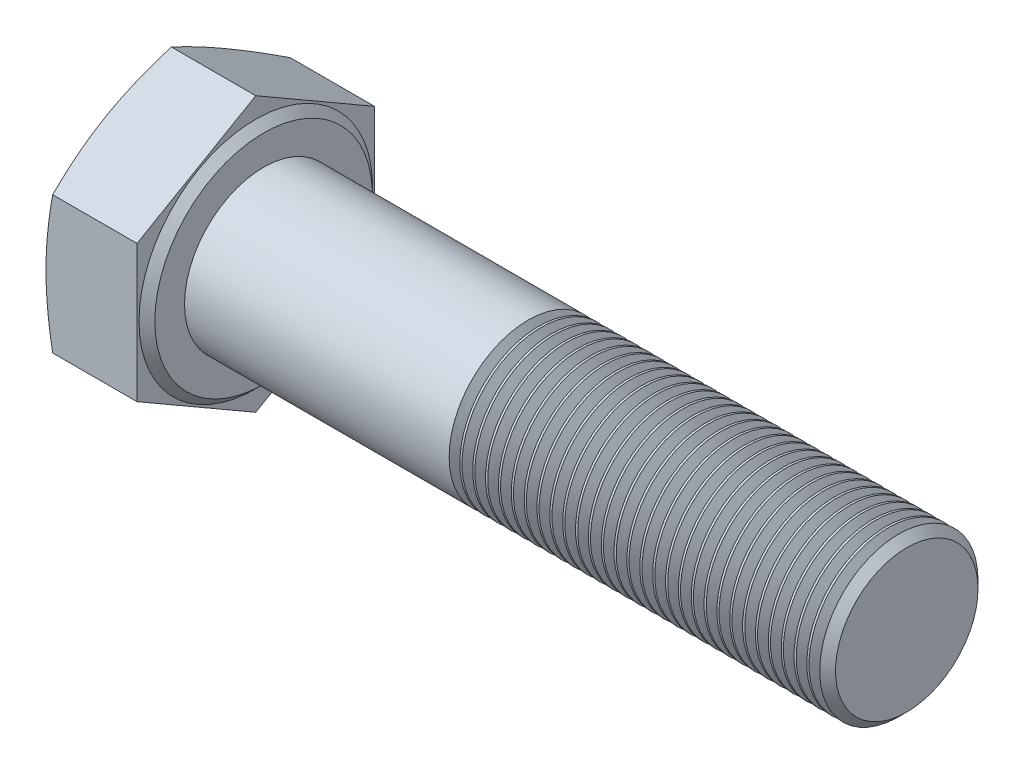
SolidWorks part; units mm, degrees
ref_plane "Front" through (0, 0, 0) normal (0, 0, 1) x (1, 0, 0)
ref_plane "Top" through (0, 0, 0) normal (0, 1, 0) x (1, 0, 0)
ref_plane "Right" through (0, 0, 0) normal (1, 0, 0) x (0, 0, -1)
other "Configuration Table"
sketch "Sketch2" plane through (0, 0, 0) normal (1, 0, 0) x (0, 0, -1)
  line L1 (0, -13.8564) -> (12, -6.9282)
  line L2 (12, -6.9282) -> (12, 6.9282)
  line L3 (12, 6.9282) -> (0, 13.8564)
  line L4 (0, 13.8564) -> (-12, 6.9282)
  line L5 (-12, 6.9282) -> (-12, -6.9282)
  line L6 (-12, -6.9282) -> (0, -13.8564)
  circle A0 centre (0, 0) radius 12 construction
extrude "BaseHead" add sketch "Sketch2" along normal blind 10
sketch "Sketch3" plane through (0, 0, 0) normal (0, 0, 1) x (1, 0, 0)
  line L0 (10, 13.8564) -> (10, 11)
  line L2 (10, 11) -> (9.2, 11.8)
  line L3 (9.2, 11.8) -> (9.2, 13.8564)
  line L5 (9.2, 13.8564) -> (10, 13.8564)
  line L6 (-0.9571, 0) -> (7.6478, 0) construction
  line L7 (10, 13.8564) -> (0, 13.8564) construction
  dimension "D1" = 45
  dimension "c" = 0.8
  dimension "dw" = 22
revolve "BearingFace" cut sketch "Sketch3" angle 360 about L6
sketch "Sketch4" plane through (0, 0, 0) normal (0, 0, 1) x (1, 0, 0)
  line L0 (-0.4935, 0) -> (3.5626, 0) construction
  line L2 (0, 13.8564) -> (0.6757, 13.8564)
  line L4 (0.6757, 13.8564) -> (0, 12)
  line L6 (0, 12) -> (0, 13.8564)
  line L7 (9.2, 13.8564) -> (0, 13.8564) construction
revolve "HeadChamfer" cut sketch "Sketch4" angle 360 about L0
ref_plane "Plane1" through (37, 0, 0) normal (1, 0, 0) x (0, 0, -1)
sketch "Sketch5" plane through (10, 0, 0) normal (1, 0, 0) x (0, 0, -1)
  circle A0 centre (0, 0) radius 8
extrude "BaseBody" add sketch "Sketch5" along normal blind 65
cosmetic thread "ThreadCosmetic1" [suppressed] parameters "D1"=38, "D2"=13.835
chamfer "Chamfer1" distance 0.8 angle 45 1 edges at (75, 0, -8)
fillet "HeadFillet" [suppressed] radius 0.6
sketch "Sketch6" plane through (0, 0, 0) normal (0, 0, 1) x (1, 0, 0)
  line L0 (73.1175, 9.0825) -> (74.2, 9.0825)
  line L1 (74.2, 9.0825) -> (74.2, 8)
  line L2 (74.2, 8) -> (73.6588, 7.0625)
  line L3 (73.6588, 7.0625) -> (73.1175, 8)
  line L4 (73.1175, 8) -> (73.1175, 9.0825)
  line L5 (74.2, -8) -> (74.2, 8) construction
  line L6 (74.2, 8) -> (10, 8) construction
revolve "Cut-Revolve10" cut sketch "Sketch6" angle 360 about axis through (75, 0, 0) along (-1, 0, 0)
pattern_linear "LPattern10" count 29 spacing 1.299 along (-1, 0, 0) of "Cut-Revolve10"
equation "\"D2@Sketch4\" = \"s@Sketch2\""
equation "\"D1@Chamfer1\" = 0.05 * \"d@Sketch5\""
equation "\"D1@ThreadCosmetic1\" = \"l@BaseBody\" - \"lg@Plane1\""
equation "\"D1@Sketch6\" =  ( \"d@Sketch5\" - \"D2@ThreadCosmetic1\" )  / 2"
equation "\"pitch@LPattern10\" = 1.2 * \"D1@Sketch6\""
equation "\"D1@LPattern10\" = \"D1@ThreadCosmetic1\" / \"pitch@LPattern10\""
